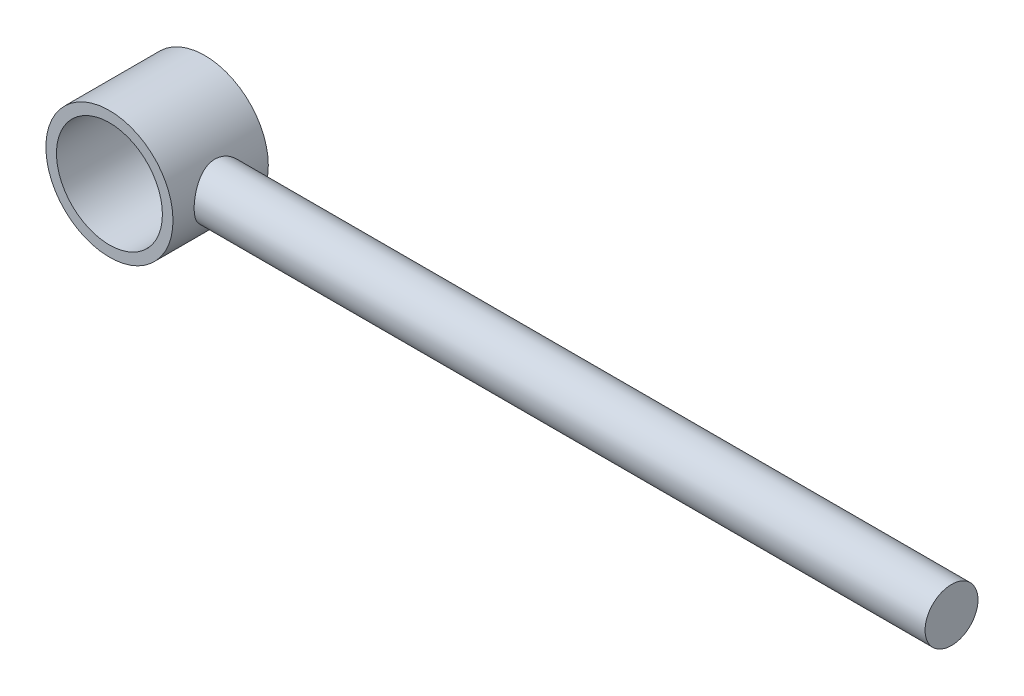
from build123d import *

# Parameters (mm, degrees)
SKETCH1_R                = 12
SKETCH1_R_2              = 10
BOSS_EXTRUDE1_DEPTH      = 9
BOSS_EXTRUDE2_REACH      = 164.693
BOSS_EXTRUDE2_END_RADIUS = 12
SKETCH2_R                = 5


with BuildPart() as part:
    # Sketch1 → Boss-Extrude1 (new, symmetric)
    with BuildSketch(Plane.XY):
        Circle(SKETCH1_R)
        Circle(SKETCH1_R_2, mode=Mode.SUBTRACT)
    extrude(amount=BOSS_EXTRUDE1_DEPTH, both=True)

    # Boss-Extrude2: up to this cylinder (the profile starts outside it)
    boss_extrude2_end = Plane(origin=(0, 0, 0), z_dir=(0, 0, -1)) * Cylinder(BOSS_EXTRUDE2_END_RADIUS, 354.386, mode=Mode.PRIVATE)
    # Sketch2 → Boss-Extrude2 (add, up to the surface)
    with BuildSketch(Plane(origin=(150, 0, 0), x_dir=(0, 0, -1), z_dir=(1, 0, 0)), mode=Mode.PRIVATE) as boss_extrude2_sk1:
        Circle(SKETCH2_R)
    boss_extrude2_tool1 = extrude(boss_extrude2_sk1.sketch, amount=-BOSS_EXTRUDE2_REACH, mode=Mode.PRIVATE) - boss_extrude2_end
    add(boss_extrude2_tool1.solids().sort_by_distance((150, 0, 0))[0])


solid = part.part
